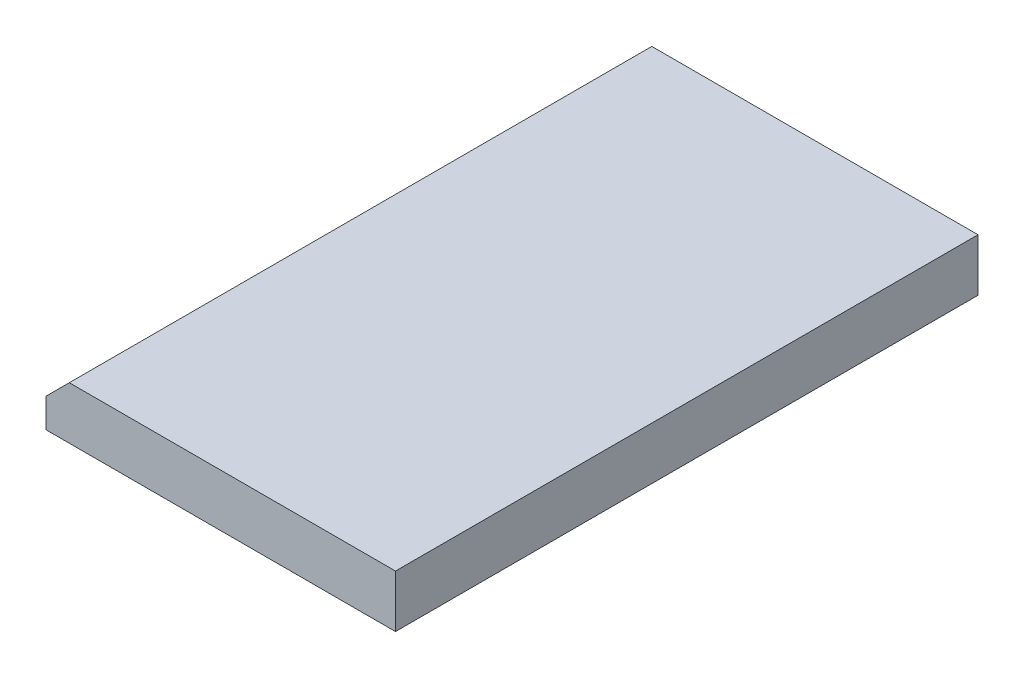
from build123d import *

# Parameters (mm, degrees)
SKETCH1_W               = 12
SKETCH1_H               = 20
BOSS_EXTRUDE2_DEPTH     = 1.8
CUT_EXTRUDE1_DEPTH      = 12.8
CUT_EXTRUDE1_DEPTH_BACK = 12.8


with BuildPart() as part:
    # Sketch1 → Boss-Extrude2 (new body)
    with BuildSketch(Plane(origin=(0, 0, 0), x_dir=(1, 0, 0), z_dir=(0, 1, 0))):
        Rectangle(SKETCH1_W, SKETCH1_H)
    extrude(amount=BOSS_EXTRUDE2_DEPTH)

    # Sketch2 → Cut-Extrude1 (cut, two sides: drawn at the far end of the back side and taken through both)
    with BuildSketch(Plane.XY.offset(-CUT_EXTRUDE1_DEPTH_BACK)):
        Polygon((-6, 1), (-5.2, 1.8), (-6, 1.8), align=None)
    extrude(amount=CUT_EXTRUDE1_DEPTH + CUT_EXTRUDE1_DEPTH_BACK, mode=Mode.SUBTRACT)


solid = part.part
